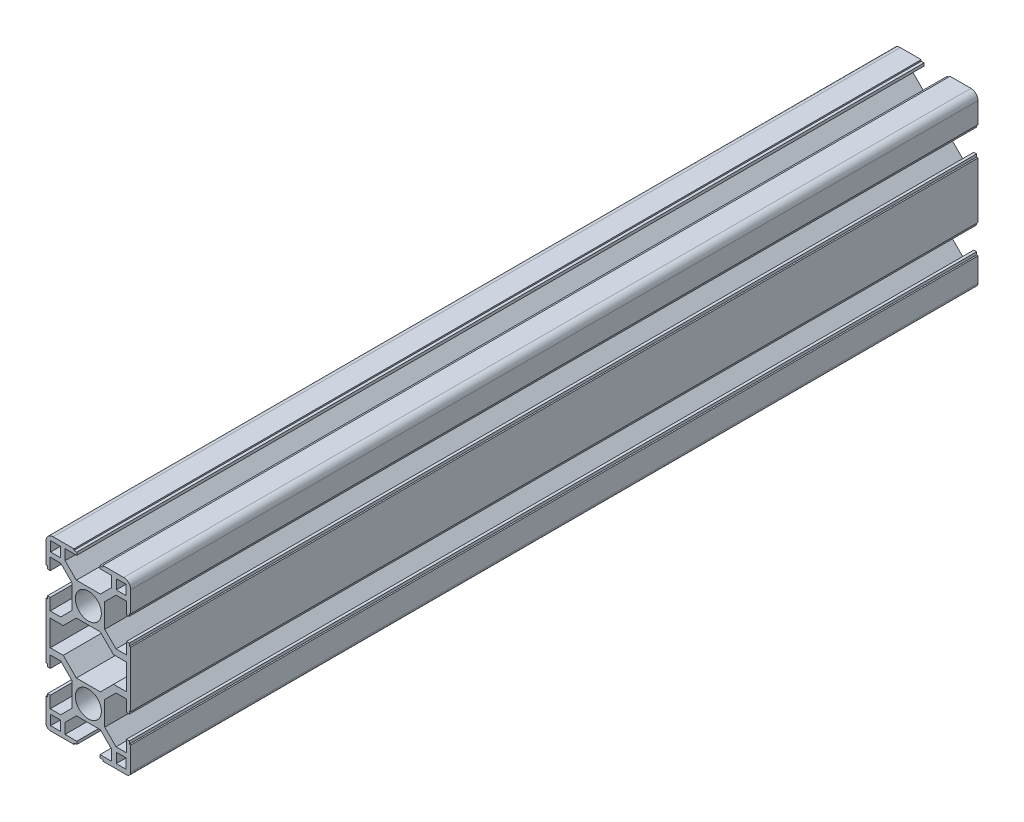
SolidWorks part; units mm, degrees
material "A6061 T6"
ref_plane "前视基准面" through (0, 0, 0) normal (0, 0, 1) x (1, 0, 0)
ref_plane "上视基准面" through (0, 0, 0) normal (0, 1, 0) x (1, 0, 0)
ref_plane "右视基准面" through (0, 0, 0) normal (1, 0, 0) x (0, 0, -1)
sketch "草图1" plane through (0, 0, 0) normal (0, 1, 0) x (1, 0, 0)
  line L0 (0, 0) -> (0, 300)
  dimension "D1" = 300
other "铝型材 30 X 60L X R2.5(1)"
ref_plane "基准面1" through (0, 0, 0) normal (0, 0, -1) x (-1, 0, 0)
sketch "Sketch1" plane through (0, 0, 0) normal (0, 0, -1) x (-1, 0, 0)
  line L0 (-5.1, 15) -> (-5.1, 14.5)
  line L1 (-5.1, 14.5) -> (-4.1, 14.5)
  line L2 (-4.1, 14.5) -> (-4.1, 13.5)
  line L3 (-4.1, 13.5) -> (-8.25, 13.5)
  line L4 (8.9, -10.45) -> (4.25, -5.8)
  line L5 (-15, -24.9) -> (-15, -5.1)
  line L6 (12.5, 15) -> (5.1, 15)
  line L7 (15, 12.5) -> (15, 5.1)
  line L8 (0, 15) -> (0, 0) construction
  line L9 (0, 0) -> (15, 0) construction
  line L10 (-8.25, 13.5) -> (-8.25, 9.8)
  line L11 (-8.25, 9.8) -> (-4.25, 5.8)
  line L12 (-4.25, 5.8) -> (4.25, 5.8)
  line L13 (8.25, 9.8) -> (4.25, 5.8)
  line L14 (8.25, 13.5) -> (8.25, 9.8)
  line L15 (4.1, 13.5) -> (8.25, 13.5)
  line L16 (4.1, 14.5) -> (4.1, 13.5)
  line L17 (5.1, 14.5) -> (4.1, 14.5)
  line L18 (5.1, 15) -> (5.1, 14.5)
  line L19 (-5.1, 15) -> (-12.5, 15)
  line L20 (15, 5.1) -> (14.5, 5.1)
  line L21 (14.5, 5.1) -> (14.5, 4.1)
  line L22 (14.5, 4.1) -> (13.5, 4.1)
  line L23 (13.5, 4.1) -> (13.5, 8.25)
  line L24 (13.5, 8.25) -> (9.8, 8.25)
  line L25 (9.8, 8.25) -> (5.8, 4.25)
  line L26 (5.8, 4.25) -> (5.8, -4.25)
  line L27 (9.8, -8.25) -> (5.8, -4.25)
  line L28 (13.5, -8.25) -> (9.8, -8.25)
  line L29 (13.5, -4.1) -> (13.5, -8.25)
  line L30 (14.5, -4.1) -> (13.5, -4.1)
  line L31 (14.5, -5.1) -> (14.5, -4.1)
  line L32 (15, -5.1) -> (14.5, -5.1)
  line L33 (8.9, -19.55) -> (4.25, -24.2)
  line L34 (-8.9, -19.55) -> (-4.25, -24.2)
  line L35 (-8.9, -10.45) -> (-4.25, -5.8)
  line L36 (-13.5, -10.45) -> (-8.9, -10.45)
  line L37 (-13.5, -19.55) -> (-8.9, -19.55)
  line L38 (-13.5, -10.45) -> (-9.8, -10.45) construction
  line L39 (4.25, -5.8) -> (-4.25, -5.8)
  line L40 (-13.5, -19.55) -> (-9.8, -19.55) construction
  line L41 (-13.5, -10.45) -> (-13.5, -19.55)
  line L42 (13.5, -10.45) -> (13.5, -19.55)
  line L43 (8.9, -10.45) -> (13.5, -10.45)
  line L44 (8.9, -19.55) -> (13.5, -19.55)
  line L45 (-11.625, 11.625) -> (-11.625, 16.245) construction
  line L46 (-15, -5.1) -> (-14.5, -5.1)
  line L47 (-14.5, -5.1) -> (-14.5, -4.1)
  line L48 (-14.5, -4.1) -> (-13.5, -4.1)
  line L49 (-13.5, -4.1) -> (-13.5, -8.25)
  line L50 (-13.5, -8.25) -> (-9.8, -8.25)
  line L51 (-9.8, -8.25) -> (-5.8, -4.25)
  line L52 (-5.8, -4.25) -> (-5.8, 4.25)
  line L53 (-9.8, 8.25) -> (-5.8, 4.25)
  line L54 (-13.5, 8.25) -> (-9.8, 8.25)
  line L55 (-13.5, 4.1) -> (-13.5, 8.25)
  line L56 (-14.5, 4.1) -> (-13.5, 4.1)
  line L57 (-14.5, 5.1) -> (-14.5, 4.1)
  line L58 (-15, 5.1) -> (-14.5, 5.1)
  line L59 (-13.375, 13.375) -> (-9.875, 13.375)
  line L60 (-15, 5.1) -> (-15, 12.5)
  line L61 (15, -5.1) -> (15, -24.9)
  line L62 (-13.375, 13.375) -> (-13.375, 9.875)
  line L63 (-13.375, 9.875) -> (-9.875, 9.875)
  line L64 (-9.875, 13.375) -> (-9.875, 9.875)
  line L65 (-11.625, 11.625) -> (-7.4229, 11.625) construction
  line L66 (-13.5, -45) -> (-5.1, -45)
  line L67 (-15, -43.5) -> (-15, -35.1)
  line L68 (9.875, 13.375) -> (13.375, 13.375)
  line L69 (9.875, 13.375) -> (9.875, 9.875)
  line L70 (9.875, 9.875) -> (13.375, 9.875)
  line L71 (13.375, 13.375) -> (13.375, 9.875)
  line L72 (-4.25, -24.2) -> (4.25, -24.2)
  line L73 (-13.375, -39.875) -> (-9.875, -39.875)
  line L74 (-13.375, -39.875) -> (-13.375, -43.375)
  line L75 (-13.375, -43.375) -> (-9.875, -43.375)
  line L76 (-9.875, -39.875) -> (-9.875, -43.375)
  line L77 (9.875, -39.875) -> (13.375, -39.875)
  line L78 (9.875, -39.875) -> (9.875, -43.375)
  line L79 (9.875, -43.375) -> (13.375, -43.375)
  line L80 (15, -24.9) -> (14.5, -24.9)
  line L81 (14.5, -24.9) -> (14.5, -25.9)
  line L82 (14.5, -25.9) -> (13.5, -25.9)
  line L83 (13.5, -25.9) -> (13.5, -21.75)
  line L84 (13.5, -21.75) -> (9.8, -21.75)
  line L85 (9.8, -21.75) -> (5.8, -25.75)
  line L86 (5.8, -25.75) -> (5.8, -34.25)
  line L87 (9.8, -38.25) -> (5.8, -34.25)
  line L88 (13.5, -38.25) -> (9.8, -38.25)
  line L89 (13.5, -34.1) -> (13.5, -38.25)
  line L90 (14.5, -34.1) -> (13.5, -34.1)
  line L91 (14.5, -35.1) -> (14.5, -34.1)
  line L92 (15, -35.1) -> (14.5, -35.1)
  line L93 (5.1, -45) -> (5.1, -44.5)
  line L94 (5.1, -44.5) -> (4.1, -44.5)
  line L95 (4.1, -44.5) -> (4.1, -43.5)
  line L96 (4.1, -43.5) -> (8.25, -43.5)
  line L97 (8.25, -43.5) -> (8.25, -39.8)
  line L98 (8.25, -39.8) -> (4.25, -35.8)
  line L99 (4.25, -35.8) -> (-4.25, -35.8)
  line L100 (-8.25, -39.8) -> (-4.25, -35.8)
  line L101 (-8.25, -43.5) -> (-8.25, -39.8)
  line L102 (-4.1, -43.5) -> (-8.25, -43.5)
  line L103 (-4.1, -44.5) -> (-4.1, -43.5)
  line L104 (-5.1, -44.5) -> (-4.1, -44.5)
  line L105 (-5.1, -45) -> (-5.1, -44.5)
  line L106 (-15, -35.1) -> (-14.5, -35.1)
  line L107 (-14.5, -35.1) -> (-14.5, -34.1)
  line L108 (-14.5, -34.1) -> (-13.5, -34.1)
  line L109 (-13.5, -34.1) -> (-13.5, -38.25)
  line L110 (-13.5, -38.25) -> (-9.8, -38.25)
  line L111 (-9.8, -38.25) -> (-5.8, -34.25)
  line L112 (-5.8, -34.25) -> (-5.8, -25.75)
  line L113 (-9.8, -21.75) -> (-5.8, -25.75)
  line L114 (-13.5, -21.75) -> (-9.8, -21.75)
  line L115 (-13.5, -25.9) -> (-13.5, -21.75)
  line L116 (-14.5, -25.9) -> (-13.5, -25.9)
  line L117 (-14.5, -24.9) -> (-14.5, -25.9)
  line L118 (-15, -24.9) -> (-14.5, -24.9)
  line L119 (5.1, -45) -> (13.5, -45)
  line L120 (13.375, -39.875) -> (13.375, -43.375)
  line L121 (15, -35.1) -> (15, -43.5)
  line L122 (0, -30) -> (15, -30) construction
  line L125 (5.1, -15) -> (5.1, -14.5) [skipped]
  line L127 (5.1, -14.5) -> (4.1, -14.5) [skipped]
  line L129 (4.1, -14.5) -> (4.1, -13.5) [skipped]
  line L131 (4.1, -13.5) -> (8.25, -13.5) [skipped]
  line L133 (-4.1, -13.5) -> (-8.25, -13.5) [skipped]
  line L135 (-4.1, -14.5) -> (-4.1, -13.5) [skipped]
  line L137 (-5.1, -14.5) -> (-4.1, -14.5) [skipped]
  line L139 (-5.1, -15) -> (-5.1, -14.5) [skipped]
  line L141 (-5.1, -15) -> (-5.1, -15.5) [skipped]
  line L142 (-5.1, -15.5) -> (-4.1, -15.5) [skipped]
  line L143 (-4.1, -15.5) -> (-4.1, -16.5) [skipped]
  line L144 (-4.1, -16.5) -> (-8.25, -16.5) [skipped]
  line L145 (12.5, -15) -> (5.1, -15) [skipped]
  line L146 (4.1, -16.5) -> (8.25, -16.5) [skipped]
  line L147 (4.1, -15.5) -> (4.1, -16.5) [skipped]
  line L148 (5.1, -15.5) -> (4.1, -15.5) [skipped]
  line L149 (5.1, -15) -> (5.1, -15.5) [skipped]
  line L150 (-5.1, -15) -> (-12.5, -15) [skipped]
  line L151 (-15, -24.9) -> (-15, -17.5) [skipped]
  line L152 (15, -17.5) -> (15, -24.9) [skipped]
  line L154 (-8.25, -13.5) -> (-8.25, -9.8) [skipped]
  line L156 (8.25, -13.5) -> (8.25, -9.8) [skipped]
  line L157 (8.25, -16.5) -> (8.25, -20.2) [skipped]
  line L158 (-8.25, -16.5) -> (-8.25, -20.2) [skipped]
  line L160 (-12.5, -14.05) -> (-9.7895, -11.3395) [skipped]
  line L161 (18.444, -10.006) -> (14.8, -13.65) [skipped]
  line L163 (11.9857, -13.5357) -> (9.7894, -11.3394) [skipped]
  line L164 (-15.9344, -12.5156) -> (-14.8, -13.65) [skipped]
  line L165 (9.7894, -15) -> (-9.8, -15) construction
  circle A0 centre (0, 0) radius 4.6
  arc A1 (-15, 12.5) -> (-12.5, 15) centre (-12.5, 12.5) cw
  arc A2 (15, 12.5) -> (12.5, 15) centre (12.5, 12.5) ccw
  arc A3 (15, -43.5) -> (13.5, -45) centre (13.5, -43.5) cw
  arc A4 (-15, -43.5) -> (-13.5, -45) centre (-13.5, -43.5) ccw
  circle A5 centre (0, -30) radius 4.6
  arc A12 (-15, -17.5) -> (-12.5, -15) centre (-12.5, -17.5) cw [skipped]
  arc A13 (15, -17.5) -> (12.5, -15) centre (12.5, -17.5) ccw [skipped]
  point P0 (-10, 0)
  point P1 (10, 0)
  point P2 (0, 20)
  point P4 (0, 0)
  point P5 (0, 0)
  point P6 (-10, 0)
  point P7 (15, 15)
  point P8 (-15, 15)
  point P12 (-15, -15)
  point P13 (15, -15)
  point P15 (0, -10)
  point P16 (10, 0)
  point P36 (-15, 15)
  point P39 (15, 15)
  point P43 (-10, -30)
  point P44 (10, -30)
  point P88 (0, -30)
  point P89 (0, -30)
  point P90 (-10, -30)
  point P91 (10, -30)
  point P102 (15, -45)
  point P120 (-15, -45)
  point P121 (0, 0)
  dimension "D1" = 16.5
  dimension "D2" = 30
  dimension "D3" = 8.2
  dimension "D4" = 10.2
  dimension "D5" = 9.2
  dimension "D6" = 9.2
  dimension "D7" = 2.5
  dimension "D8" = 45
  dimension "D14" = 30
  dimension "D15" = 1.5
  dimension "D9" = 0.5
  dimension "D10" = 1
  dimension "D11" = 8.5
  dimension "D12" = 15
  dimension "D13" = 60
  dimension "D16" = 45
  dimension "D17" = 45
  dimension "D18" = 10.2
  dimension "D19" = 8.2
  dimension "D20" = 2.2
  dimension "D22" = 3.5
  dimension "D21" = 2.2
